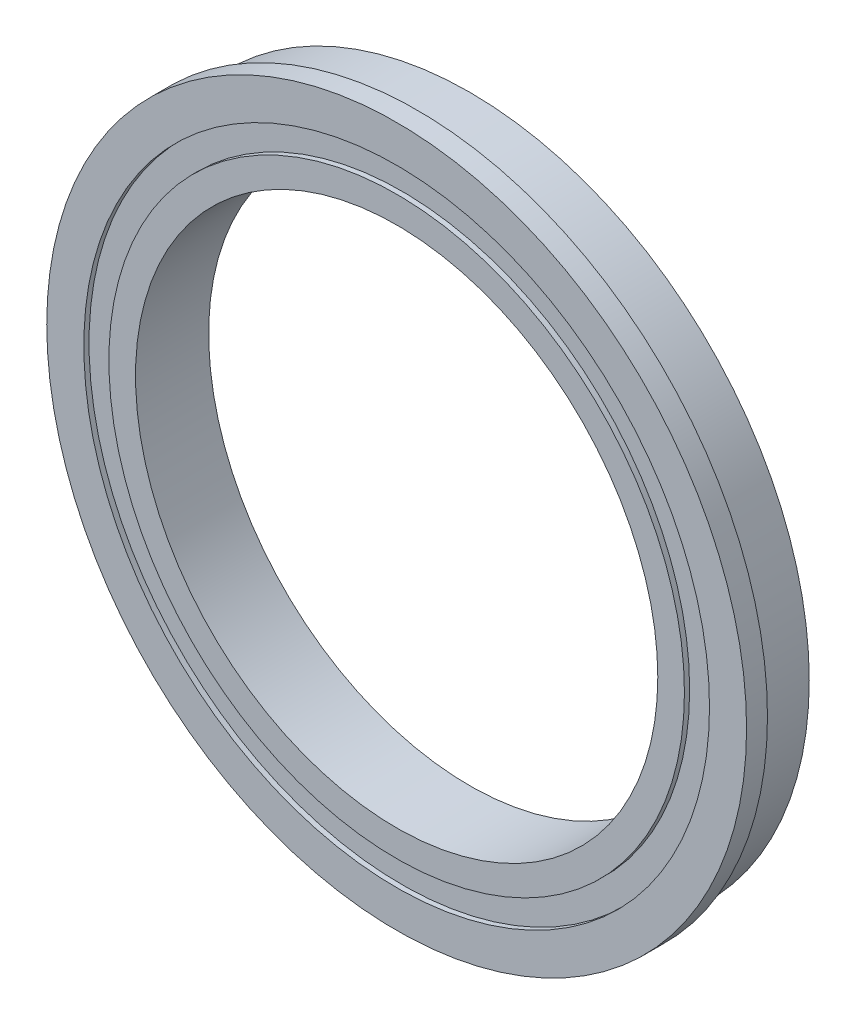
SolidWorks part; units mm, degrees
material "合金钢"
ref_plane "前视基准面" through (0, 0, 0) normal (0, 0, 1) x (1, 0, 0)
ref_plane "上视基准面" through (0, 0, 0) normal (0, 1, 0) x (1, 0, 0)
ref_plane "右视基准面" through (0, 0, 0) normal (1, 0, 0) x (0, 0, -1)
other "Configuration Table"
sketch "草图1" plane through (0, 0, 0) normal (1, 0, 0) x (0, 0, -1)
  line L0 (0, 0) -> (89.3968, 0) construction
  line L1 (-3.5, 25) -> (-3.5, 27.55)
  line L2 (-3.5, 27.55) -> (-3, 27.55)
  line L3 (-3, 27.55) -> (-3, 29.95)
  line L4 (-3, 29.95) -> (-3.5, 29.95)
  line L5 (-3.5, 29.95) -> (-3.5, 32.5)
  line L6 (-3.5, 32.5) -> (3.5, 32.5)
  line L7 (0, 32.5) -> (0, 25) construction
  line L8 (3.5, 25) -> (-3.5, 25)
  line L9 (3.5, 25) -> (3.5, 27.55)
  line L10 (3.5, 27.55) -> (3, 27.55)
  line L11 (3, 27.55) -> (3, 29.95)
  line L12 (3, 29.95) -> (3.5, 29.95)
  line L13 (3.5, 29.95) -> (3.5, 32.5)
  dimension "D1" = 25
  dimension "D2" = 27.55
  dimension "D3" = 29.95
  dimension "D4" = 32.5
  dimension "D5" = 3.5
  dimension "D6" = 0.5
revolve "旋转1" add sketch "草图1" angle 360 about L0
sketch "草图2" plane through (0, 0, 3.5) normal (0, 0, 1) x (1, 0, 0)
  circle A0 centre (0, 0) radius 33.5
  circle A1 centre (0, 0) radius 32.5 construction
  circle A2 centre (0, 0) radius 32.5
  dimension "D1" = 67
extrude "凸台-拉伸1" add sketch "草图2" against normal blind 2
